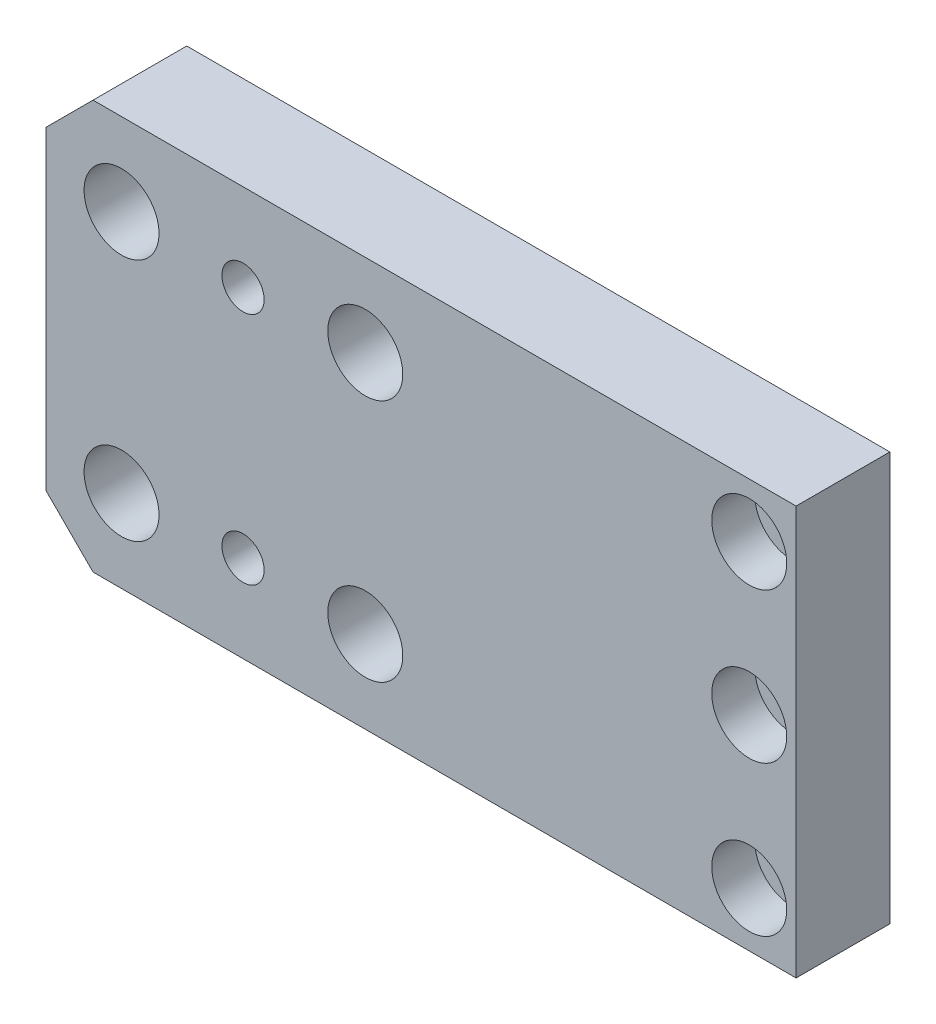
from build123d import *

# Parameters (mm, degrees)
SKETCH_1_W                   = 80
SKETCH_1_H                   = 10
EXTRUDE_1_DEPTH              = 43.6
CHAMFER_1_SIZE               = 5
HOLE_WIZARD_8_0_8_1_D        = 8
HOLE_WIZARD_M4_1_D           = 4.5
HOLE_WIZARD_M4_1_CBORE_D     = 8
HOLE_WIZARD_M4_1_CBORE_DEPTH = 4.6
HOLE_WIZARD_M4_2_D           = 4.5
HOLE_WIZARD_M4_2_CBORE_D     = 8
HOLE_WIZARD_M4_2_CBORE_DEPTH = 4.6


with BuildPart() as part:
    # 草图1 → 凸台-拉伸1 (new body)
    with BuildSketch(Plane(origin=(0, 0, 0), x_dir=(1, 0, 0), z_dir=(0, 1, 0))):
        with Locations((40, 5)):
            Rectangle(SKETCH_1_W, SKETCH_1_H)
    extrude(amount=EXTRUDE_1_DEPTH)

    # 倒角1
    chamfer_1_edges = [part.edges().sort_by_distance(p)[0] for p in [
        (0, 43.6, -5),
        (0, 0, -5),
    ]]
    chamfer(chamfer_1_edges, length=CHAMFER_1_SIZE)

    # Ø8.0 (8) 直径孔1 (through all)
    with Locations(Plane(origin=(0, 0, -10), x_dir=(-1, 0, 0), z_dir=(0, 0, -1))):
        with Locations((-34.042753413, 34.8), (-8.042753413, 34.8), (-8.042753413, 8.8), (-34.042753413, 8.8)):
            Hole(HOLE_WIZARD_8_0_8_1_D / 2)

    # M4 六角圆柱头螺钉的柱形沉头孔1 (through all)
    with Locations(Plane(origin=(0, 0, -10), x_dir=(-1, 0, 0), z_dir=(0, 0, -1))):
        with Locations((-21, 34.3), (-21, 9.3)):
            CounterBoreHole(HOLE_WIZARD_M4_1_D / 2, HOLE_WIZARD_M4_1_CBORE_D / 2, HOLE_WIZARD_M4_1_CBORE_DEPTH)

    # M4 六角圆柱头螺钉的柱形沉头孔2 (through all)
    with Locations(Plane.XY):
        with Locations((75, 37.8), (75, 5.8), (75, 21.8)):
            CounterBoreHole(HOLE_WIZARD_M4_2_D / 2, HOLE_WIZARD_M4_2_CBORE_D / 2, HOLE_WIZARD_M4_2_CBORE_DEPTH)


solid = part.part
